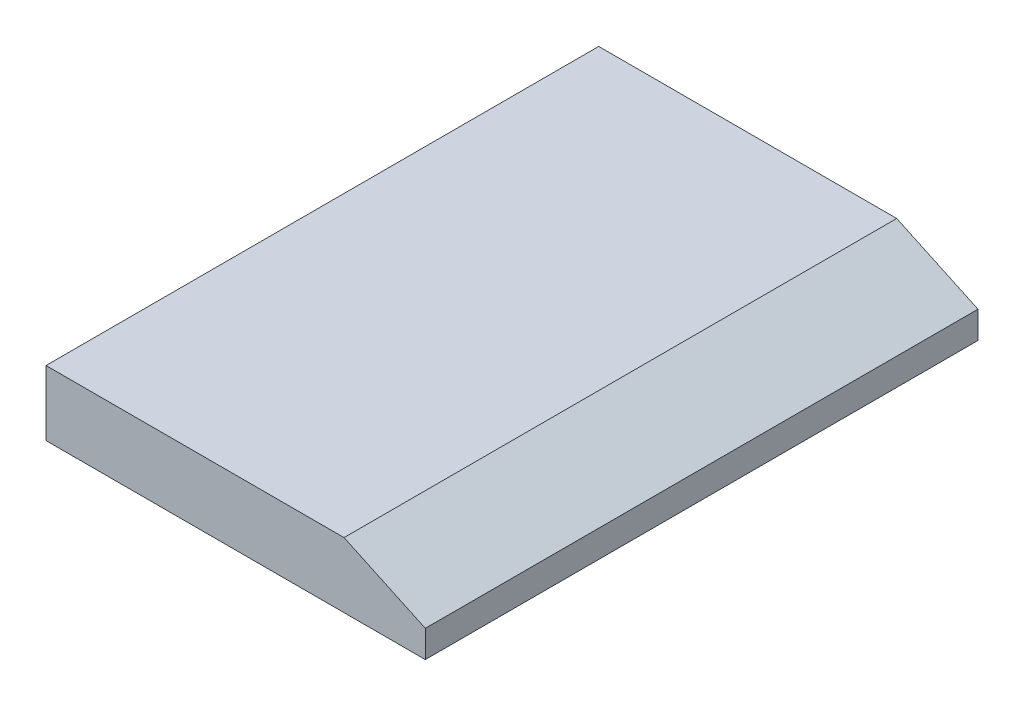
SolidWorks part; units mm, degrees
material "普通碳钢"
ref_plane "Front Plane" through (0, 0, 0) normal (0, 0, 1) x (1, 0, 0)
ref_plane "Top Plane" through (0, 0, 0) normal (0, 1, 0) x (1, 0, 0)
ref_plane "Right Plane" through (0, 0, 0) normal (1, 0, 0) x (0, 0, -1)
sketch "Sketch1" plane through (0, 0, 0) normal (0, 0, 1) x (1, 0, 0)
  line L0 (0, 0) -> (0, 5)
  line L1 (0, -55) -> (0, 55) construction
  line L2 (0, 5) -> (-15, 12)
  line L3 (-15, 12) -> (-70, 12)
  line L4 (-70, 0) -> (0, 0)
  line L5 (-70, 0) -> (-70, 12)
  dimension "D2" = 15
  dimension "D3" = 5
  dimension "D7" = 70
  dimension "D1" = 12
extrude "Boss-Extrude1" add sketch "Sketch1" along normal blind 102
